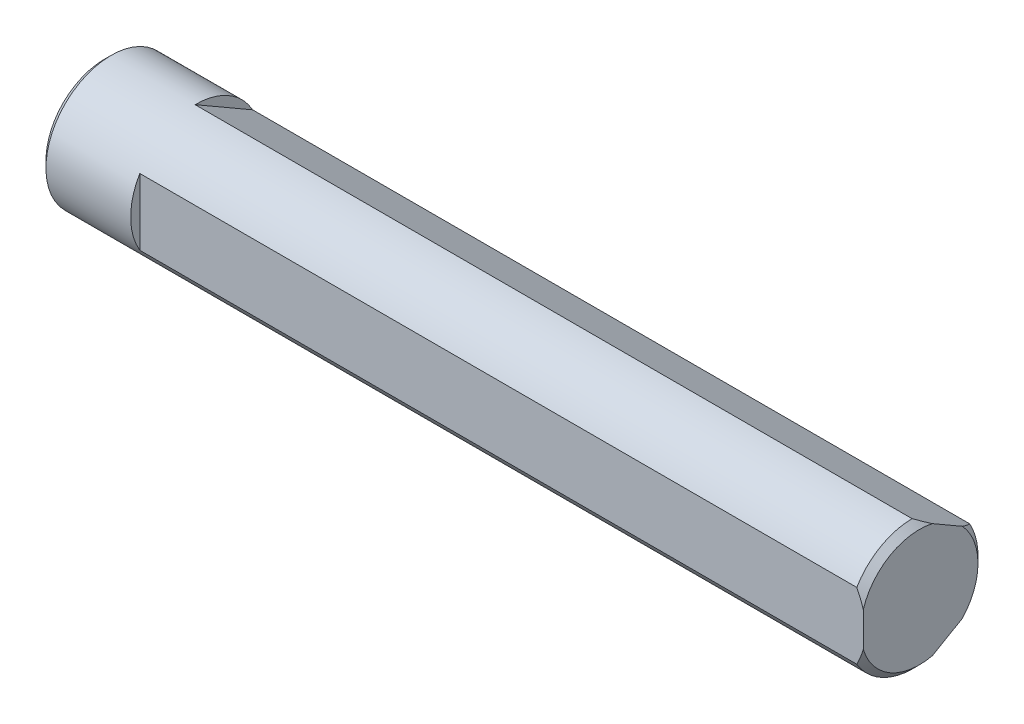
from build123d import *

# Parameters (mm, degrees)
SKETCH_1_R               = 5
EXTRUDE_1_DEPTH          = 62.5
CHAMFER_1_SIZE           = 0.5
SKETCH_2_W               = 4.472118267
SKETCH_2_H               = 12.857340018
CUT_EXTRUDE_1_DEPTH      = 55.5
PATTERN_CIRCULAR_1_COUNT = 3
HOLE_WIZARD_M4_1_D       = 3.3
HOLE_WIZARD_M4_1_DEPTH   = 15.5
HOLE_WIZARD_M4_1_TIP     = 0.991420021


with BuildPart() as part:
    # 草图1 → 凸台-拉伸1 (new body)
    with BuildSketch(Plane(origin=(0, 0, 0), x_dir=(0, 0, -1), z_dir=(1, 0, 0))):
        Circle(SKETCH_1_R)
    extrude(amount=EXTRUDE_1_DEPTH)

    # 倒角1
    chamfer_1_edges = [part.edges().sort_by_distance(p)[0] for p in [
        (0, 0, 5),
        (62.5, 0, 5),
    ]]
    chamfer(chamfer_1_edges, length=CHAMFER_1_SIZE)

    # 草图2 → 切除-拉伸1 (cut)
    with BuildSketch(Plane(origin=(62.5, 0, 0), x_dir=(0, 0, -1), z_dir=(1, 0, 0))):
        with Locations((-6.536059134, -0.104972075)):
            Rectangle(SKETCH_2_W, SKETCH_2_H)
    cut_extrude_1 = extrude(amount=-CUT_EXTRUDE_1_DEPTH, mode=Mode.SUBTRACT)

    # 阵列(圆周)1: 切除-拉伸1 ×3 about axis
    pattern_circular_1_axis = Axis((0, 0, 0), (1, 0, 0))
    for i in range(1, PATTERN_CIRCULAR_1_COUNT):
        add(cut_extrude_1.rotate(pattern_circular_1_axis, i * 360 / PATTERN_CIRCULAR_1_COUNT), mode=Mode.SUBTRACT)

    # M4 螺纹孔1
    with Locations(Plane.ZY):
        with Locations((0, 0)):
            Hole(HOLE_WIZARD_M4_1_D / 2, depth=HOLE_WIZARD_M4_1_DEPTH)
            with Locations((0, 0, -(HOLE_WIZARD_M4_1_DEPTH + HOLE_WIZARD_M4_1_TIP / 2))):  # 118° drill point
                Cone(0, HOLE_WIZARD_M4_1_D / 2, HOLE_WIZARD_M4_1_TIP, mode=Mode.SUBTRACT)


solid = part.part
